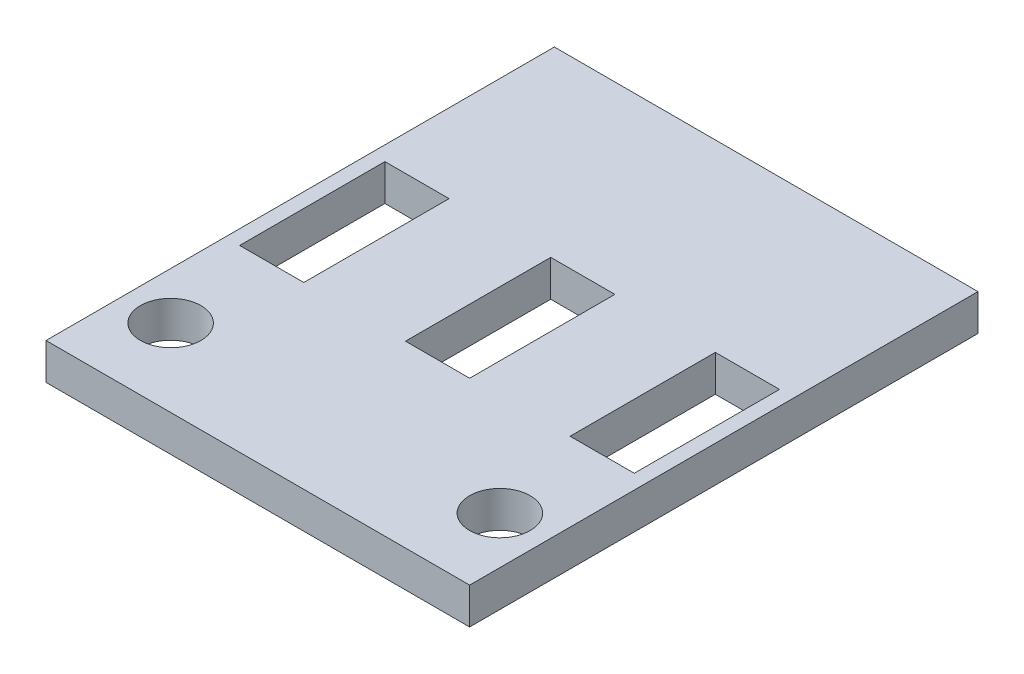
SolidWorks part; units mm, degrees
ref_plane "Front Plane" through (0, 0, 0) normal (0, 0, 1) x (1, 0, 0)
ref_plane "Top Plane" through (0, 0, 0) normal (0, 1, 0) x (1, 0, 0)
ref_plane "Right Plane" through (0, 0, 0) normal (1, 0, 0) x (0, 0, -1)
sketch "Sketch1" plane through (0, 0, 0) normal (0, 1, 0) x (1, 0, 0)
  line L0 (-24.519, 64) -> (473.2458, 64) construction
  line L1 (0, 0) -> (350, 0)
  line L2 (0, 0) -> (0, 420)
  line L3 (0, 420) -> (350, 420)
  line L4 (350, 0) -> (350, 420)
  line L5 (149, 148) -> (202, 148)
  line L6 (39, 325.2954) -> (39, -35.5409) construction
  line L7 (175, 420) -> (175, -50.2386) construction
  line L8 (311, 351.5989) -> (311, -56.4011) construction
  line L9 (149, 148) -> (149, 268)
  line L10 (149, 268) -> (202, 268)
  line L11 (202, 268) -> (202, 148)
  line L12 (285, 148) -> (338, 148)
  line L13 (285, 148) -> (285, 268)
  line L14 (285, 268) -> (338, 268)
  line L15 (338, 268) -> (338, 148)
  line L16 (12, 268) -> (12, 148)
  line L17 (65, 268) -> (12, 268)
  line L18 (65, 148) -> (65, 268)
  line L19 (65, 148) -> (12, 148)
  circle A0 centre (311, 64) radius 25
  circle A1 centre (39, 64) radius 25
  dimension "D13" = 50
  dimension "D14" = 50
  dimension "D1" = 420
  dimension "D2" = 350
  dimension "D3" = 64
  dimension "D4" = 148
  dimension "D5" = 136
  dimension "D6" = 136
  dimension "D7" = 26
  dimension "D8" = 53
  dimension "D9" = 120
  dimension "D11" = 83
  dimension "D12" = 148
  dimension "D10" = 2
extrude "Boss-Extrude1" add sketch "Sketch1" along normal blind 30
